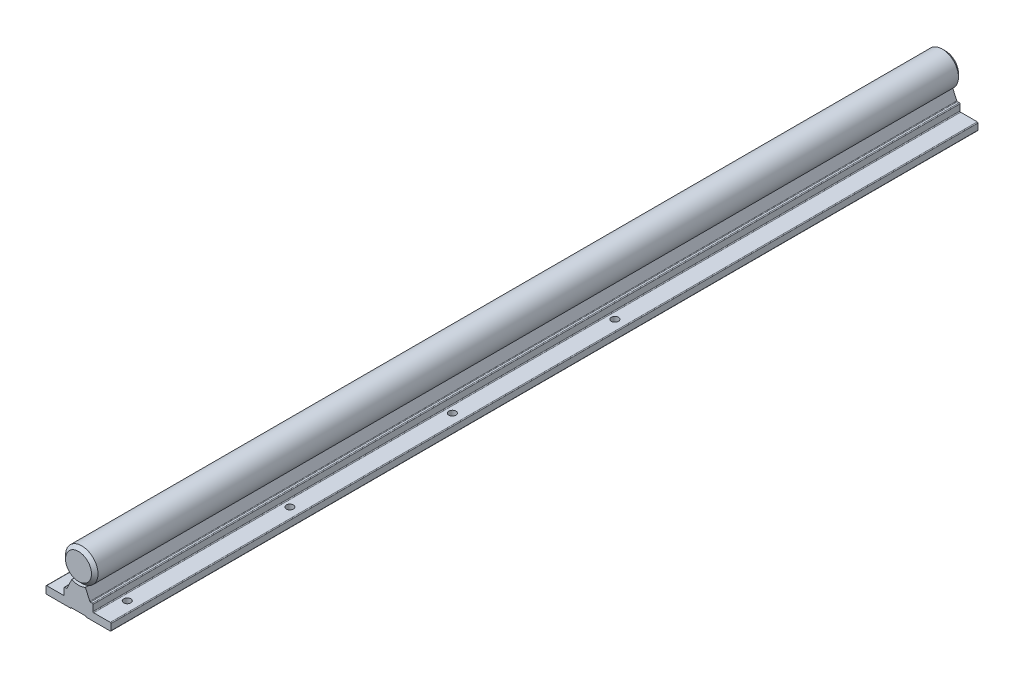
SolidWorks part; units mm, degrees
material "Plain carbon steel"
ref_plane "Front Plane" through (0, 0, 0) normal (0, 0, 1) x (1, 0, 0)
ref_plane "Top Plane" through (0, 0, 0) normal (0, 1, 0) x (1, 0, 0)
ref_plane "Right Plane" through (0, 0, 0) normal (1, 0, 0) x (0, 0, -1)
sketch "Sketch1" plane through (0, 0, 0) normal (0, 0, 1) x (1, 0, 0)
  line L0 (-60.7963, 0) -> (64.5121, 0) construction
  line L1 (0, 86.3494) -> (0, -79.6624) construction
  line L2 (-30, 0.7) -> (-30, 6.3)
  line L3 (-29.3, 7) -> (-14.06, 7)
  line L4 (-13.36, 7.7) -> (-13.36, 13.3)
  line L5 (-12.66, 14) -> (-11.1339, 14)
  line L6 (-10.4995, 14.4042) -> (-6.3088, 23.3912)
  line L7 (-29.3, 0) -> (-7, 0)
  line L8 (-7, 0) -> (-7, 0.7)
  line L9 (-7, 0.7) -> (7, 0.7)
  line L10 (-20, 7) -> (-20, 0) construction
  line L11 (20, 7) -> (20, 0) construction
  line L12 (7, 0) -> (7, 0.7)
  line L13 (29.3, 0) -> (7, 0)
  line L14 (10.4995, 14.4042) -> (6.3088, 23.3912)
  line L15 (12.66, 14) -> (11.1339, 14)
  line L16 (13.36, 7.7) -> (13.36, 13.3)
  line L17 (29.3, 7) -> (14.06, 7)
  line L18 (30, 0.7) -> (30, 6.3)
  circle A0 centre (0, 37) radius 15
  arc A1 (29.3, 0) -> (30, 0.7) centre (29.3, 0.7) ccw
  arc A2 (30, 6.3) -> (29.3, 7) centre (29.3, 6.3) ccw
  arc A3 (14.06, 7) -> (13.36, 7.7) centre (14.06, 7.7) cw
  arc A4 (13.36, 13.3) -> (12.66, 14) centre (12.66, 13.3) ccw
  arc A5 (11.1339, 14) -> (10.4995, 14.4042) centre (11.1339, 14.7) cw
  arc A6 (-10.4995, 14.4042) -> (-11.1339, 14) centre (-11.1339, 14.7) cw
  arc A7 (-12.66, 14) -> (-13.36, 13.3) centre (-12.66, 13.3) ccw
  arc A8 (-13.36, 7.7) -> (-14.06, 7) centre (-14.06, 7.7) cw
  arc A9 (-29.3, 0) -> (-30, 0.7) centre (-29.3, 0.7) cw
  arc A10 (-29.3, 7) -> (-30, 6.3) centre (-29.3, 6.3) ccw
  point P18 (-23.3, 0)
  point P19 (-16.7, 0)
  point P23 (0, 0.7)
  point P30 (16.7, 0)
  point P31 (23.3, 0)
  point P34 (30, 0)
  point P37 (30, 7)
  point P40 (13.36, 7)
  point P43 (13.36, 14)
  point P46 (10.688, 14)
  point P49 (-10.688, 14)
  point P52 (-13.36, 14)
  point P55 (-13.36, 7)
  point P58 (-30, 0)
  point P61 (-30, 7)
  dimension "D1" = 0.7
  dimension "Dr" = 30
  dimension "D6" = 0.7
  dimension "h" = 37
  dimension "B" = 60
  dimension "T" = 7
  dimension "C" = 40
  dimension "S2" = 6.6
  dimension "h1" = 14
  dimension "D3" = 26.72
  dimension "D4" = 14
  dimension "D5" = 21.376
  dimension "θ" = 50
sketch "Sketch2" plane through (0, 0, 0) normal (1, 0, 0) x (0, 0, -1)
  line L0 (0, 0) -> (25, 0) construction
  line L1 (25, 0) -> (475, 0)
  line L2 (475, 0) -> (500, 0) construction
  line L3 (0, 86.3494) -> (0, -79.6624) construction
  point P5 (225, 0)
  dimension "N" = 25
  dimension "P" = 200
  dimension "L" = 500
sketch "Sketch6" plane through (0, 0, 0) normal (0, 0, 1) x (1, 0, 0)
  circle A0 centre (0, 37) radius 15 construction
  circle A1 centre (0, 37) radius 15
extrude "Boss-Extrude2" add sketch "Sketch6" against normal blind 800
chamfer "Chamfer1" distance 3 angle 45 2 edges at (15, 37, -800) (15, 37, 0)
sketch "Sketch3" plane through (0, 0, 0) normal (0, 0, 1) x (1, 0, 0)
  line L0 (-10.4995, 14.4042) -> (-6.3088, 23.3912) construction
  line L1 (-12.66, 14) -> (-11.1339, 14) construction
  line L2 (-13.36, 7.7) -> (-13.36, 13.3) construction
  line L3 (-29.3, 7) -> (-14.06, 7) construction
  line L4 (-30, 0.7) -> (-30, 6.3) construction
  line L5 (-29.3, 0) -> (-7, 0) construction
  line L6 (-7, 0) -> (-7, 0.7) construction
  line L7 (-7, 0.7) -> (7, 0.7) construction
  line L8 (7, 0) -> (7, 0.7) construction
  line L9 (29.3, 0) -> (7, 0) construction
  line L10 (30, 0.7) -> (30, 6.3) construction
  line L11 (29.3, 7) -> (14.06, 7) construction
  line L12 (13.36, 7.7) -> (13.36, 13.3) construction
  line L13 (12.66, 14) -> (11.1339, 14) construction
  line L14 (10.4995, 14.4042) -> (6.3088, 23.3912) construction
  line L15 (-10.4995, 14.4042) -> (-6.3088, 23.3912)
  line L16 (-12.66, 14) -> (-11.1339, 14)
  line L17 (-13.36, 7.7) -> (-13.36, 13.3)
  line L18 (-29.3, 7) -> (-14.06, 7)
  line L19 (-30, 0.7) -> (-30, 6.3)
  line L20 (-29.3, 0) -> (-7, 0)
  line L21 (-7, 0) -> (-7, 0.7)
  line L22 (-7, 0.7) -> (7, 0.7)
  line L23 (7, 0) -> (7, 0.7)
  line L24 (29.3, 0) -> (7, 0)
  line L25 (30, 0.7) -> (30, 6.3)
  line L26 (29.3, 7) -> (14.06, 7)
  line L27 (13.36, 7.7) -> (13.36, 13.3)
  line L28 (12.66, 14) -> (11.1339, 14)
  line L29 (10.4995, 14.4042) -> (6.3088, 23.3912)
  circle A0 centre (0, 37) radius 15 construction
  arc A1 (-11.1339, 14) -> (-10.4995, 14.4042) centre (-11.1339, 14.7) ccw construction
  arc A2 (-12.66, 14) -> (-13.36, 13.3) centre (-12.66, 13.3) ccw construction
  arc A3 (-14.06, 7) -> (-13.36, 7.7) centre (-14.06, 7.7) ccw construction
  arc A4 (-29.3, 7) -> (-30, 6.3) centre (-29.3, 6.3) ccw construction
  arc A5 (-30, 0.7) -> (-29.3, 0) centre (-29.3, 0.7) ccw construction
  arc A6 (29.3, 0) -> (30, 0.7) centre (29.3, 0.7) ccw construction
  arc A7 (30, 6.3) -> (29.3, 7) centre (29.3, 6.3) ccw construction
  arc A8 (13.36, 7.7) -> (14.06, 7) centre (14.06, 7.7) ccw construction
  arc A9 (13.36, 13.3) -> (12.66, 14) centre (12.66, 13.3) ccw construction
  arc A10 (10.4995, 14.4042) -> (11.1339, 14) centre (11.1339, 14.7) ccw construction
  arc A11 (6.3088, 23.3912) -> (-6.3088, 23.3912) centre (0, 37) ccw construction
  arc A12 (-11.1339, 14) -> (-10.4995, 14.4042) centre (-11.1339, 14.7) ccw
  arc A13 (-12.66, 14) -> (-13.36, 13.3) centre (-12.66, 13.3) ccw
  arc A14 (-14.06, 7) -> (-13.36, 7.7) centre (-14.06, 7.7) ccw
  arc A15 (-29.3, 7) -> (-30, 6.3) centre (-29.3, 6.3) ccw
  arc A16 (-30, 0.7) -> (-29.3, 0) centre (-29.3, 0.7) ccw
  arc A17 (29.3, 0) -> (30, 0.7) centre (29.3, 0.7) ccw
  arc A18 (30, 6.3) -> (29.3, 7) centre (29.3, 6.3) ccw
  arc A19 (13.36, 7.7) -> (14.06, 7) centre (14.06, 7.7) ccw
  arc A20 (13.36, 13.3) -> (12.66, 14) centre (12.66, 13.3) ccw
  arc A21 (10.4995, 14.4042) -> (11.1339, 14) centre (11.1339, 14.7) ccw
  arc A22 (-6.3088, 23.3912) -> (6.3088, 23.3912) centre (0, 37) ccw
  point P0 (13.36, 7)
extrude "Boss-Extrude1" add sketch "Sketch3" against normal blind 800
ref_plane "Plane1" through (0, 0, -25) normal (0, 0, 1) x (1, 0, 0)
sketch "Sketch4" plane through (0, 0, -25) normal (0, 0, 1) x (1, 0, 0)
  line L0 (-23.3, 0) -> (-23.3, 7)
  line L1 (-29.3, 7) -> (-14.06, 7) construction
  line L2 (-23.3, 7) -> (-20, 7)
  line L3 (-20, 7) -> (-20, 0)
  line L4 (-20, 0) -> (-23.3, 0)
revolve "Cut-Revolve1" cut sketch "Sketch4" angle 360 about L3
mirror "Mirror1" about plane through (0, 0, 0) normal (1, 0, 0) of "Cut-Revolve1"
sketch "Sketch5" plane through (0, 0, -25) normal (0, 0, 1) x (1, 0, 0)
  line L0 (-7, 0.7) -> (-7, 9.1)
  line L1 (-7, 9.1) -> (-2.8, 9.1)
  line L2 (-2.8, 9.1) -> (-2.8, 34.4757)
  line L3 (-2.8, 34.4757) -> (0, 34.4757)
  line L4 (0, 86.3494) -> (0, -79.6624) construction
  line L5 (-29.3, 0) -> (-7, 0) construction
  line L6 (0, 34.4757) -> (0, 0.7)
  line L7 (0, 0.7) -> (-7, 0.7)
  dimension "D1" = 9.1
  dimension "D2" = 2.8
  dimension "D3" = 2.5243
revolve "Cut-Revolve2" cut sketch "Sketch5" angle 360 about L6
pattern_curve "Curve Pattern1" of "Cut-Revolve1", "Mirror1", "Cut-Revolve2" parameters "D1"=4, "D3"=10, "D2"=1, "D4"=10
sketch "Sketch7" plane through (0, 0, 0) normal (1, 0, 0) x (0, 0, -1)
  line L0 (0, 37) -> (730, 37)
  line L1 (0, 52) -> (0, 22) construction
  line L2 (800, 25) -> (800, 49) construction
  dimension "M" = 70
